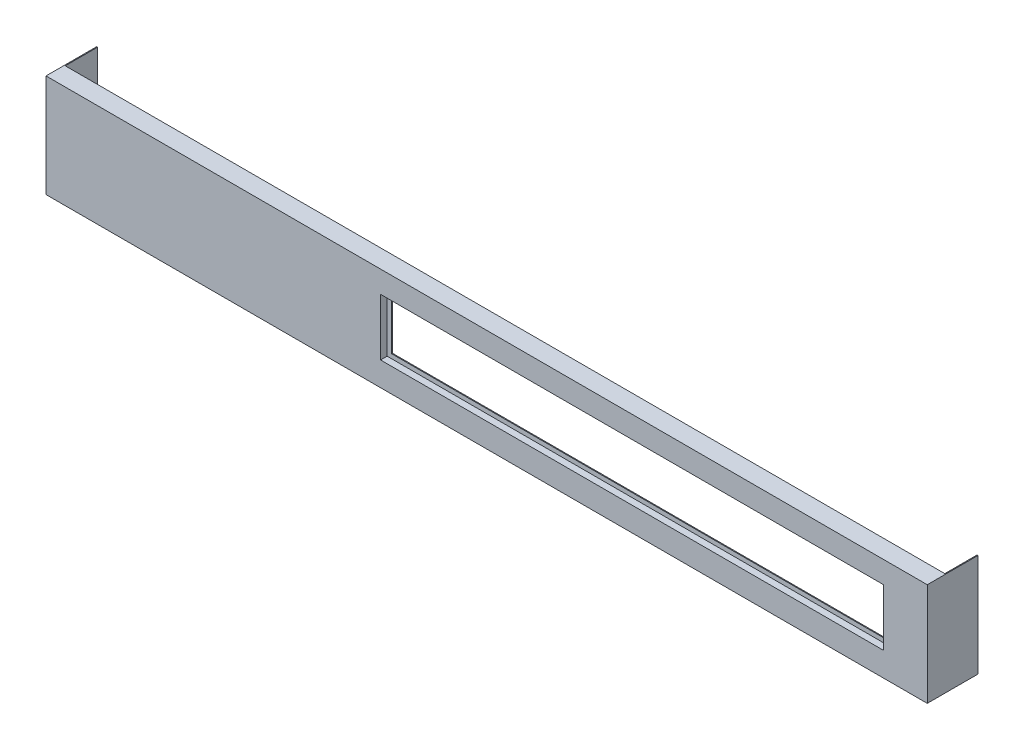
SolidWorks part; units mm, degrees
ref_plane "前视基准面" through (0, 0, 0) normal (0, 0, 1) x (1, 0, 0)
ref_plane "上视基准面" through (0, 0, 0) normal (0, 1, 0) x (1, 0, 0)
ref_plane "右视基准面" through (0, 0, 0) normal (1, 0, 0) x (0, 0, -1)
sketch "草图2" plane through (0, 0, 0) normal (0, 0, 1) x (1, 0, 0)
  line L1 (0, 0) -> (2015, 0)
  line L2 (0, 0) -> (0, 235)
  line L3 (0, 235) -> (2015, 235)
  line L4 (2015, 0) -> (2015, 235)
  dimension "D1" = 235
  dimension "D2" = 2015
extrude "凸台-拉伸1" add sketch "草图2" along normal blind 2
sketch "草图3" plane through (0, 0, 0) normal (0, 0, -1) x (-1, 0, 0)
  line L0 (0, 0) -> (-2015, 0) construction
  line L1 (-2015, 235) -> (-2013, 235)
  line L2 (-2015, 235) -> (-2015, 0)
  line L3 (-2015, 0) -> (-2013, 0)
  line L4 (-2013, 235) -> (-2013, 0)
  line L5 (-1007.5, 235) -> (-1007.5, -229.1775) construction
  line L6 (-2015, 235) -> (0, 235) construction
  line L7 (-2, 235) -> (-2, 0)
  line L8 (0, 0) -> (-2, 0)
  line L9 (0, 235) -> (0, 0)
  line L10 (0, 235) -> (-2, 235)
  dimension "D1" = 2
extrude "凸台-拉伸2" add sketch "草图3" along normal blind 114
sketch "草图4" plane through (0, 0, 0) normal (0, 0, -1) x (-1, 0, 0)
  line L0 (-2, 235) -> (-2, 0) construction
  line L1 (-2013, 235) -> (-2, 235)
  line L2 (-2013, 235) -> (-2013, 233)
  line L3 (-2013, 233) -> (-2, 233)
  line L4 (-2, 235) -> (-2, 233)
  dimension "D1" = 2
extrude "凸台-拉伸3" add sketch "草图4" along normal blind 40
sketch "草图5" plane through (0, 0, 2) normal (0, 0, 1) x (1, 0, 0)
  line L0 (2015, 235) -> (0, 235) construction
  line L1 (1915, 55) -> (765, 55)
  line L2 (1915, 55) -> (1915, 185)
  line L3 (1915, 185) -> (765, 185)
  line L4 (765, 55) -> (765, 185)
  line L5 (2015, 0) -> (2015, 235) construction
  dimension "D1" = 50
  dimension "D2" = 100
  dimension "D3" = 1150
  dimension "D4" = 130
extrude "切除-拉伸1" cut sketch "草图5" against normal blind 10
sketch "草图6" plane through (0, 0, 0) normal (0, -1, 0) x (1, 0, 0)
  line L0 (2015, 2) -> (2015, -114) construction
  line L1 (0, 2) -> (2015, 2)
  line L2 (0, 2) -> (0, -40)
  line L3 (0, -40) -> (2015, -40)
  line L4 (2015, 2) -> (2015, -40)
extrude "凸台-拉伸4" add sketch "草图6" against normal blind 2
sketch "草图7" plane through (0, 0, 0) normal (0, 0, -1) x (-1, 0, 0)
  line L10 (-1917, 187) -> (-1917, 53)
  line L11 (-1917, 53) -> (-763, 53)
  line L12 (-763, 53) -> (-763, 187)
  line L13 (-763, 187) -> (-1917, 187)
  line L14 (-765, 55) -> (-765, 185)
  line L15 (-1915, 55) -> (-765, 55)
  line L16 (-765, 185) -> (-1915, 185)
  line L17 (-1915, 185) -> (-1915, 55)
  line L18 (-765, 55) -> (-765, 185)
  line L19 (-1915, 55) -> (-765, 55)
  line L20 (-765, 185) -> (-1915, 185)
  line L21 (-1915, 185) -> (-1915, 55)
  dimension "D1" = 0
  dimension "D2" = 2
extrude "凸台-拉伸5" add sketch "草图7" along normal blind 15
sketch "草图8" plane through (0, 0, -15) normal (0, 0, -1) x (-1, 0, 0)
  line L0 (-763, 53) -> (-763, 187) construction
  line L1 (-1917, 187) -> (-763, 187)
  line L2 (-1917, 187) -> (-1917, 53)
  line L3 (-1917, 53) -> (-763, 53)
  line L4 (-763, 187) -> (-763, 53)
  line L5 (-1915, 55) -> (-765, 55) construction
  line L20 (-1905, 175) -> (-1905, 65)
  line L21 (-775, 175) -> (-1905, 175)
  line L22 (-775, 65) -> (-775, 175)
  line L23 (-1905, 65) -> (-775, 65)
  line L24 (-1905, 175) -> (-1905, 65)
  line L25 (-775, 175) -> (-1905, 175)
  line L26 (-775, 65) -> (-775, 175)
  line L27 (-1905, 65) -> (-775, 65)
  dimension "D1" = 2
  dimension "D2" = 10
extrude "凸台-拉伸6" add sketch "草图8" against normal blind 2
